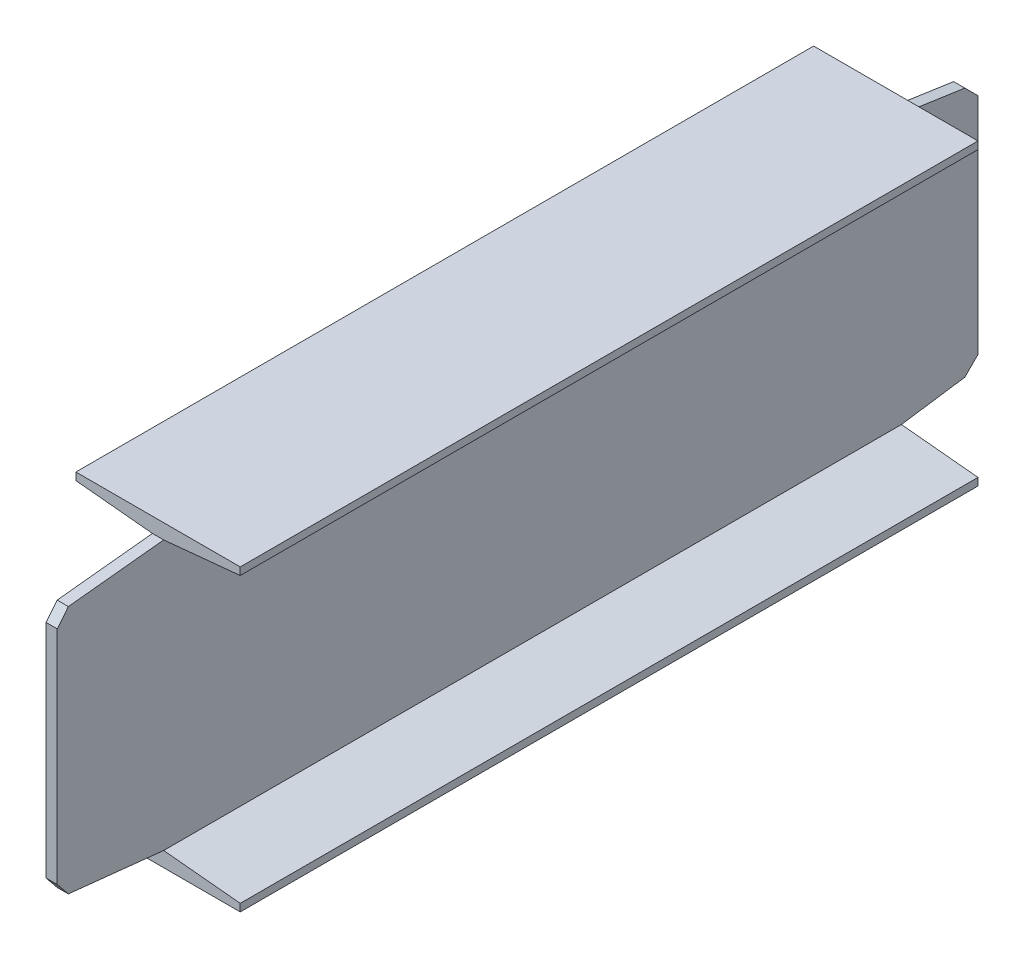
from build123d import *
from OCP.BRepFilletAPI import BRepFilletAPI_MakeChamfer

# Parameters (mm, degrees)
EXTRUDE_1_DEPTH          = 246.5
CUT_EXTRUDE_1_DEPTH      = 263.865459884
CUT_EXTRUDE_1_DEPTH_BACK = 263.865459884
CHAMFER_1_SIZE           = 6
CHAMFER_1_SIZE2          = 7.103434065
CHAMFER_1_SIZE2_2        = 6.742931709


with BuildPart() as part:
    # 草图1 → 凸台-拉伸1 (new, symmetric)
    with BuildSketch(Plane.XY):
        Polygon((44, 80), (-44, 80), (-44, 76), (-3, 72), (-3, -72), (-44, -76), (-44, -80), (44, -80), (44, -76), (3, -72), (3, 72), (44, 76), align=None)
    extrude(amount=EXTRUDE_1_DEPTH, both=True)

    # 草图3 → 切除-拉伸1 (cut, two sides: drawn at the far end of the back side and taken through both)
    with BuildSketch(Plane(origin=(0, 0, 0), x_dir=(0, 0, -1), z_dir=(1, 0, 0)).offset(-CUT_EXTRUDE_1_DEPTH_BACK)):
        Polygon((-246.5, 66), (-189.5, 72), (-189.5, 80), (-246.5, 80), align=None)
        Polygon((246.5, 80), (246.5, 66), (205.5, 72), (205.5, 80), align=None)
        Polygon((246.5, -66), (205.5, -72), (205.5, -80), (246.5, -80), align=None)
        Polygon((-246.5, -80), (-246.5, -66), (-189.5, -72), (-189.5, -80), align=None)
    extrude(amount=CUT_EXTRUDE_1_DEPTH + CUT_EXTRUDE_1_DEPTH_BACK, mode=Mode.SUBTRACT)

    # 倒角1: one chamfer whose edges measure the first distance from different faces: ONE call of the kernel's chamfer builder (chamfer() names one face for all edges)
    chamfer_1_edges_1 = [part.edges().sort_by_distance(p)[0] for p in [
        (0, 66, -246.5),
        (0, -66, -246.5),
    ]]
    chamfer_1_side_1 = [part.faces().sort_by_distance(p)[0] for p in [
        (0, 0, -246.5),
    ]]
    chamfer_1_edges_2 = [part.edges().sort_by_distance(p)[0] for p in [
        (0, 66, 246.5),
    ]]
    chamfer_1_side_2 = [part.faces().sort_by_distance(p)[0] for p in [
        (0, 69, 218),
    ]]
    chamfer_1_edges_3 = [part.edges().sort_by_distance(p)[0] for p in [
        (0, -66, 246.5),
    ]]
    chamfer_1_side_3 = [part.faces().sort_by_distance(p)[0] for p in [
        (0, -69, 218),
    ]]
    chamfer_1 = BRepFilletAPI_MakeChamfer(part.part.solid().wrapped)
    for e in chamfer_1_edges_1:
        chamfer_1.Add(CHAMFER_1_SIZE, CHAMFER_1_SIZE2, e.wrapped, chamfer_1_side_1[0].wrapped)  # the first distance lies on this face
    for e in chamfer_1_edges_2:
        chamfer_1.Add(CHAMFER_1_SIZE, CHAMFER_1_SIZE2_2, e.wrapped, chamfer_1_side_2[0].wrapped)  # the first distance lies on this face
    for e in chamfer_1_edges_3:
        chamfer_1.Add(CHAMFER_1_SIZE, CHAMFER_1_SIZE2_2, e.wrapped, chamfer_1_side_3[0].wrapped)  # the first distance lies on this face
    add(Compound.cast(chamfer_1.Shape()), mode=Mode.REPLACE)


solid = part.part
